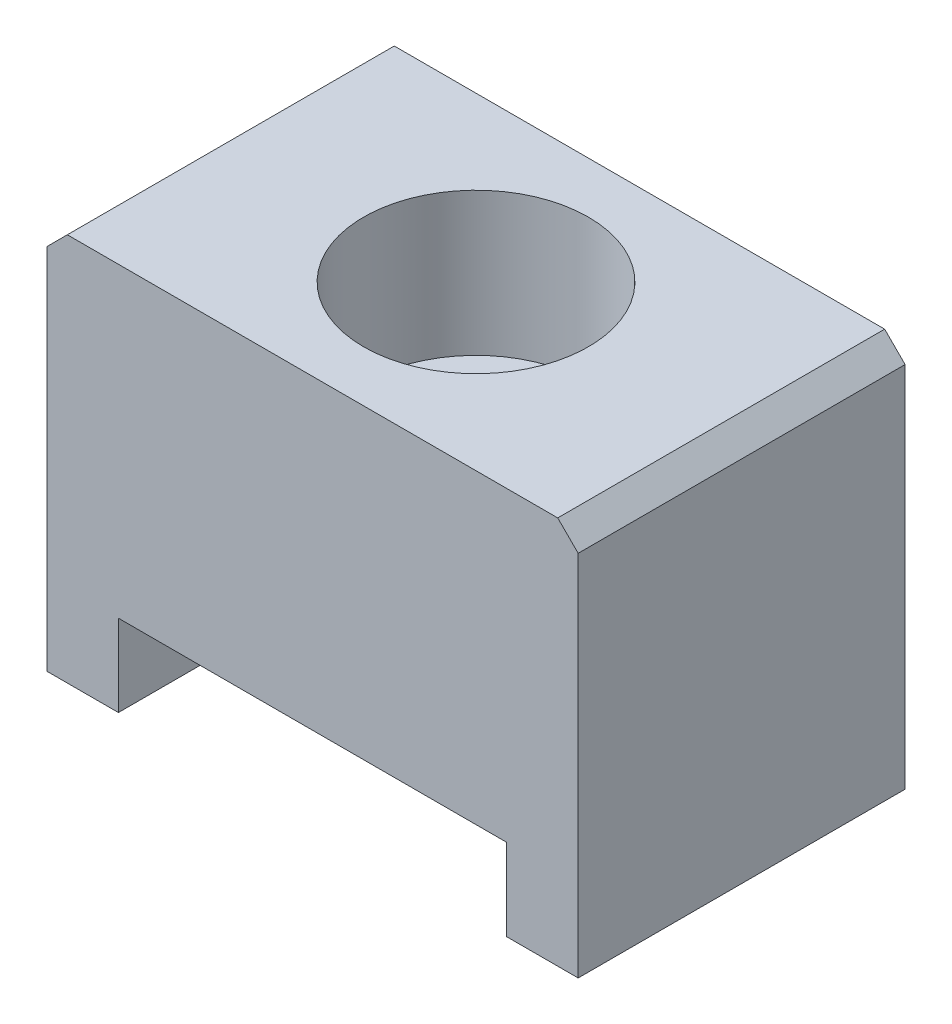
SolidWorks part; units mm, degrees
material "AISI 1045 钢，冷拔"
ref_plane "Front Plane" through (0, 0, 0) normal (0, 0, 1) x (1, 0, 0)
ref_plane "Top Plane" through (0, 0, 0) normal (0, 1, 0) x (1, 0, 0)
ref_plane "Right Plane" through (0, 0, 0) normal (1, 0, 0) x (0, 0, -1)
sketch "Sketch1" plane through (0, 0, 0) normal (0, 0, 1) x (1, 0, 0)
  line L0 (0, 0) -> (0, 19)
  line L1 (0, 19) -> (26, 19)
  line L2 (26, 19) -> (26, 0)
  line L3 (26, 0) -> (22.5, 0)
  line L4 (22.5, 0) -> (22.5, 4)
  line L5 (22.5, 4) -> (3.5, 4)
  line L6 (3.5, 4) -> (3.5, 0)
  line L7 (3.5, 0) -> (0, 0)
  dimension "D1" = 26
  dimension "D2" = 19
  dimension "D3" = 3.5
  dimension "D4" = 3.5
  dimension "D5" = 15
extrude "Boss-Extrude1" add sketch "Sketch1" along normal blind 16
ref_plane "Plane1" through (0, 19, 0) normal (0, 1, 0) x (1, 0, 0)
sketch "Sketch2" plane through (0, 19, 0) normal (0, 1, 0) x (1, 0, 0)
  line L0 (0, -8) -> (26, -8) construction
  line L1 (0, -16) -> (0, 0) construction
  line L2 (26, -16) -> (26, 0) construction
  circle A0 centre (13, -8) radius 5.5
extrude "Cut-Extrude1" cut sketch "Sketch2" against normal blind 7
ref_plane "Plane2" through (0, 12, 0) normal (0, 1, 0) x (1, 0, 0)
sketch "Sketch3" plane through (0, 12, 0) normal (0, 1, 0) x (1, 0, 0)
  circle A0 centre (13, -8) radius 3.5
extrude "Cut-Extrude2" cut sketch "Sketch3" against normal blind 8
chamfer "Chamfer1" distance 1 2 edges at (26, 19, 8) (0, 19, 8)
